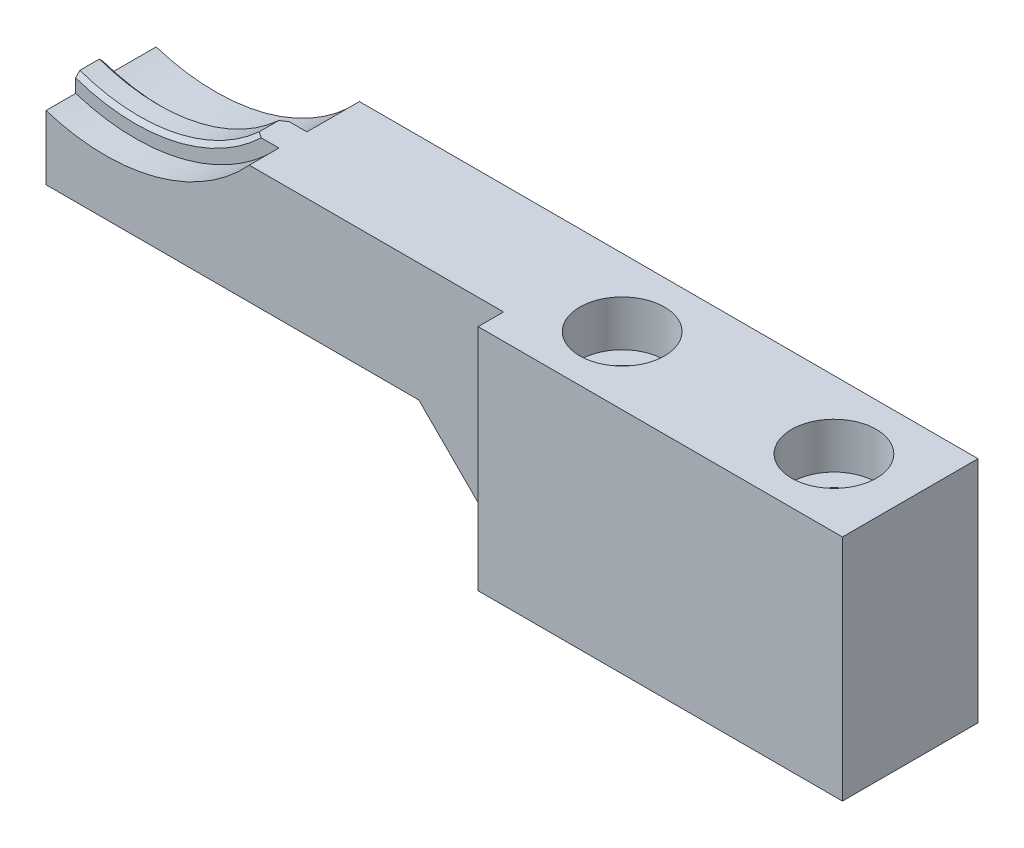
from build123d import *

# Parameters (mm, degrees)
SKETCH_1_W                   = 115
SKETCH_1_H                   = 19
EXTRUDE_1_DEPTH              = 7.5
SKETCH_2_W                   = 72
SKETCH_2_H                   = 19
EXTRUDE_2_DEPTH              = 15
SKETCH_5_R                   = 23
CUT_EXTRUDE_3_DEPTH          = 6.5
CUT_EXTRUDE_START            = -9.2
SKETCH_6_R                   = 23
CUT_EXTRUDE_4_DEPTH          = 9.2
SKETCH_7_R                   = 21
CUT_EXTRUDE_5_DEPTH          = 63.998015842
FILLET_3_R                   = 2
CHAMFER_1_SIZE               = 0.5
SKETCH_8_W                   = 100
SKETCH_8_H                   = 30
CUT_EXTRUDE_8_DEPTH          = 3
SKETCH_12_W                  = 43
SKETCH_12_H                  = 3
CUT_EXTRUDE_9_DEPTH          = 61.178899957
SKETCH_13_W                  = 72
SKETCH_13_H                  = 13
CUT_EXTRUDE_10_DEPTH         = 64.099128362
SKETCH_14_W                  = 43
SKETCH_14_H                  = 15
EXTRUDE_3_DEPTH              = 16
SKETCH_16_W                  = 115
SKETCH_16_H                  = 3
CUT_EXTRUDE_14_DEPTH         = 64.784794426
CHAMFER_2_SIZE               = 10
HOLE_WIZARD_M5_1_D           = 5.5
HOLE_WIZARD_M5_1_CBORE_D     = 10
HOLE_WIZARD_M5_1_CBORE_DEPTH = 5.4
SKETCH_19_W                  = 25.462348227
SKETCH_19_H                  = 32.507755261
CUT_EXTRUDE_15_DEPTH         = 63.789330304


with BuildPart() as part:
    # 草图1 → 凸台-拉伸1 (new, symmetric)
    with BuildSketch(Plane(origin=(0, 0, 0), x_dir=(1, 0, 0), z_dir=(0, 1, 0))):
        Rectangle(SKETCH_1_W, SKETCH_1_H)
    extrude(amount=EXTRUDE_1_DEPTH, both=True)

    # 草图2 → 凸台-拉伸2 (add)
    with BuildSketch(Plane(origin=(0, 7.5, 0), x_dir=(1, 0, 0), z_dir=(0, 1, 0))):
        with Locations((-21.5, 0)):
            Rectangle(SKETCH_2_W, SKETCH_2_H)
    extrude(amount=EXTRUDE_2_DEPTH)

    # 草图5 → 切除-拉伸3 (cut)
    with BuildSketch(Plane.XY.offset(9.5)):
        with Locations((-32.5, 35)):
            Circle(SKETCH_5_R)
    extrude(amount=-CUT_EXTRUDE_3_DEPTH, mode=Mode.SUBTRACT)

    # 草图6 → 切除-拉伸4 (cut)
    with BuildSketch(Plane(origin=(0, 0, -9.5), x_dir=(-1, 0, 0), z_dir=(0, 0, -1)).offset(CUT_EXTRUDE_START)):
        with Locations((32.5, 35)):
            Circle(SKETCH_6_R)
    extrude(amount=CUT_EXTRUDE_4_DEPTH, mode=Mode.SUBTRACT)

    # 草图7 → 切除-拉伸5 (cut, through all)
    with BuildSketch(Plane.XY.offset(3)):
        with Locations((-32.5, 35)):
            Circle(SKETCH_7_R)
    extrude(amount=-CUT_EXTRUDE_5_DEPTH, mode=Mode.SUBTRACT)

    # 圆角3
    fillet_3_edges = [part.edges().sort_by_distance(p)[0] for p in [
        (-49.374537031, 22.5, 1.35),
        (-15.625462969, 22.5, 1.35),
    ]]
    fillet(fillet_3_edges, radius=FILLET_3_R)

    # 倒角1
    chamfer_1_edges = [part.edges().sort_by_distance(p)[0] for p in [
        (-51.080152824, 22.5, 3),
        (-13.919847176, 22.5, -0.3),
        (-32.5, 14, 3),
        (-32.5, 14, -0.3),
        (-51.080152824, 22.5, -0.3),
        (-49.493844118, 22.305787796, -0.3),
        (-15.506155882, 22.305787796, -0.3),
        (-13.919847176, 22.5, 3),
        (-49.493844118, 22.305787796, 3),
        (-15.506155882, 22.305787796, 3),
    ]]
    chamfer(chamfer_1_edges, length=CHAMFER_1_SIZE)

    # 草图8 → 切除-拉伸8 (cut)
    with BuildSketch(Plane.XY.offset(9.5)):
        with Locations((-35.5, 7.5)):
            Rectangle(SKETCH_8_W, SKETCH_8_H)
    cut_extrude_8 = extrude(amount=-CUT_EXTRUDE_8_DEPTH, mode=Mode.SUBTRACT)

    # 镜向1: 切除-拉伸8 across plane
    add(cut_extrude_8.mirror(Plane.XY), mode=Mode.SUBTRACT)

    # 草图12 → 切除-拉伸9 (cut, through all)
    with BuildSketch(Plane(origin=(0, 7.5, 0), x_dir=(1, 0, 0), z_dir=(0, 1, 0))):
        with Locations((36, 8)):
            Rectangle(SKETCH_12_W, SKETCH_12_H)
    extrude(amount=-CUT_EXTRUDE_9_DEPTH, mode=Mode.SUBTRACT)

    # 草图13 → 切除-拉伸10 (cut, through all)
    with BuildSketch(Plane.XY.offset(6.5)):
        with Locations((-21.5, -1)):
            Rectangle(SKETCH_13_W, SKETCH_13_H)
    extrude(amount=-CUT_EXTRUDE_10_DEPTH, mode=Mode.SUBTRACT)

    # 草图14 → 凸台-拉伸3 (add)
    with BuildSketch(Plane.XY.offset(9.5)):
        with Locations((36, 15)):
            Rectangle(SKETCH_14_W, SKETCH_14_H)
    extrude(amount=-EXTRUDE_3_DEPTH)

    # 草图16 → 切除-拉伸14 (cut, through all)
    with BuildSketch(Plane.XY.offset(9.5)):
        with Locations((0, 21)):
            Rectangle(SKETCH_16_W, SKETCH_16_H)
    extrude(amount=-CUT_EXTRUDE_14_DEPTH, mode=Mode.SUBTRACT)

    # 倒角2
    chamfer_2_edges = [part.edges().sort_by_distance(p)[0] for p in [
        (14.5, 5.5, 0),
    ]]
    chamfer(chamfer_2_edges, length=CHAMFER_2_SIZE)

    # M5 六角凹头螺钉的柱形沉头孔1 (through all)
    with Locations(Plane(origin=(0, 19.5, 0), x_dir=(1, 0, 0), z_dir=(0, 1, 0))):
        with Locations((23.5, -1.5), (48.5, -1.5)):
            CounterBoreHole(HOLE_WIZARD_M5_1_D / 2, HOLE_WIZARD_M5_1_CBORE_D / 2, HOLE_WIZARD_M5_1_CBORE_DEPTH)

    # 草图19 → 切除-拉伸15 (cut, through all)
    with BuildSketch(Plane(origin=(0, 0, -6.5), x_dir=(-1, 0, 0), z_dir=(0, 0, -1))):
        with Locations((52.231174114, 11.069476533)):
            Rectangle(SKETCH_19_W, SKETCH_19_H)
    extrude(amount=-CUT_EXTRUDE_15_DEPTH, mode=Mode.SUBTRACT)


solid = part.part
